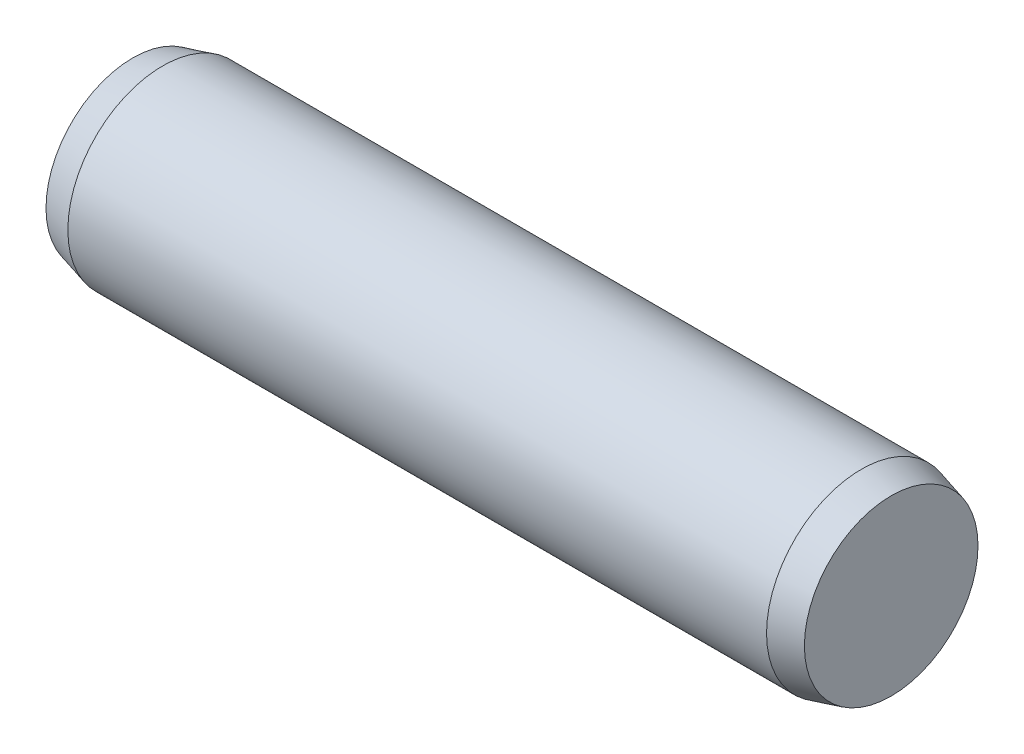
from build123d import *


with BuildPart() as part:
    # Sketch1 → Base-Revolve (revolve)
    with BuildSketch(Plane.XY, mode=Mode.PRIVATE) as base_revolve_sk:
        Polygon((-1.63, 0), (14.37, 0), (14.37, 1.831192009), (13.74, 2), (-1, 2), (-1.63, 1.831192009), align=None)
    revolve(base_revolve_sk.sketch.rotate(Axis((0, 0, 0), (1, 0, 0)), 90), axis=Axis((0, 0, 0), (1, 0, 0)))


solid = part.part
